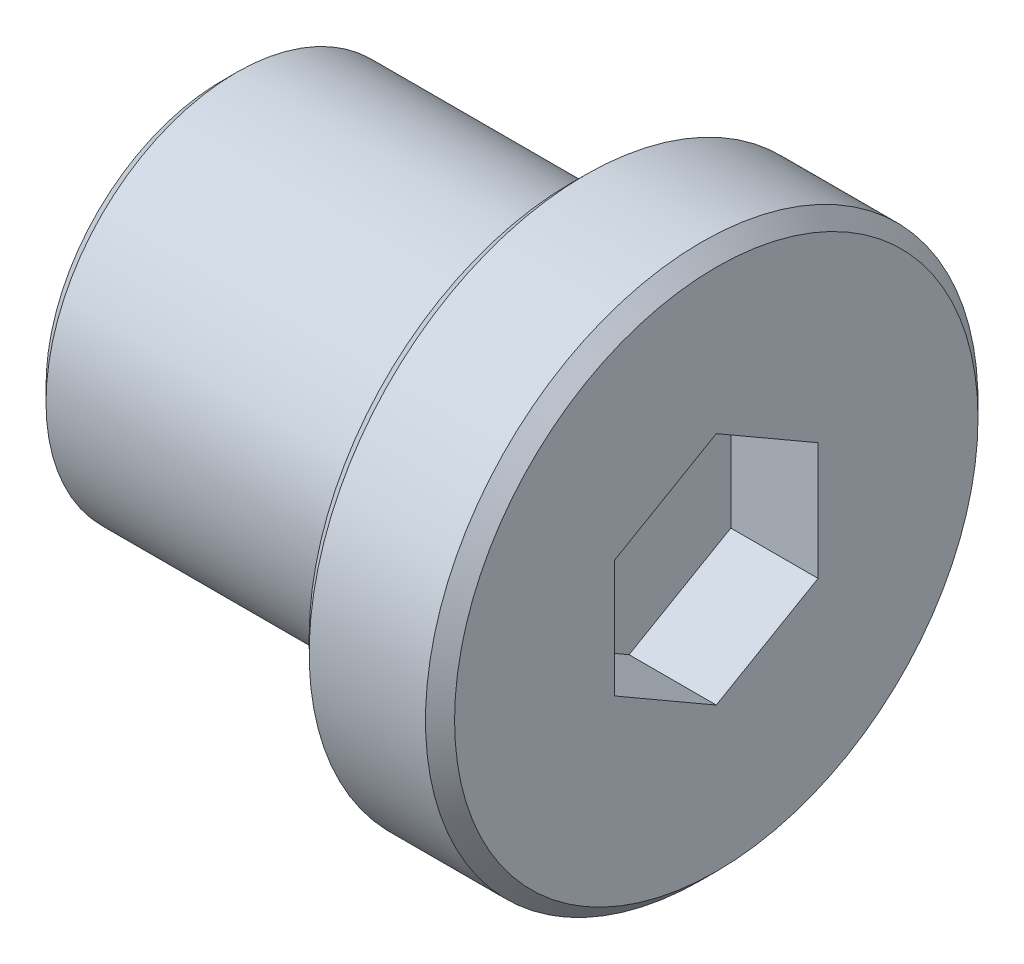
from build123d import *

# Parameters (mm, degrees)
CUT_EXTRUDE1_DEPTH = 3
CHAMFER1_SIZE      = 0.5


with BuildPart() as part:
    # Sketch1 → Revolve1 (revolve)
    with BuildSketch(Plane.XY):
        Polygon((0, 0), (0, 6.55), (12, 6.55), (12, 9.5), (17, 9.5), (17, 0), align=None)
    revolve(axis=Axis((17, 0, 0), (-1, 0, 0)))

    # Sketch2 → Cut-Extrude1 (cut)
    with BuildSketch(Plane(origin=(17, 0, 0), x_dir=(0, 0, -1), z_dir=(1, 0, 0))):
        Polygon((0, 4.041451884), (-3.5, 2.020725942), (-3.5, -2.020725942), (0, -4.041451884), (3.5, -2.020725942), (3.5, 2.020725942), align=None)
    extrude(amount=-CUT_EXTRUDE1_DEPTH, mode=Mode.SUBTRACT)

    # Chamfer1
    chamfer1_edges = [part.edges().sort_by_distance(p)[0] for p in [
        (17, -9.5, 0),
        (12, -9.5, 0),
        (0, -6.55, 0),
    ]]
    chamfer(chamfer1_edges, length=CHAMFER1_SIZE)


solid = part.part
